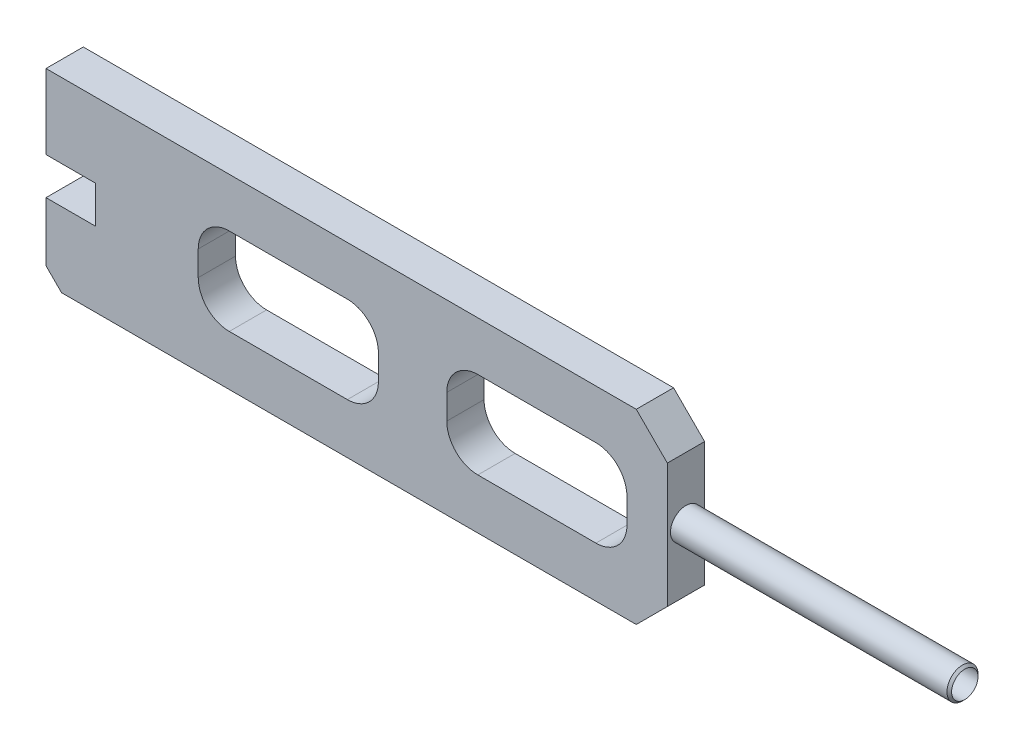
from build123d import *

# Parameters (mm, degrees)
SKETCH1_W              = 200
SKETCH1_H              = 60
BOSS_EXTRUDE1_DEPTH    = 12
SKETCH2_W              = 16
SKETCH2_H              = 12
CUT_EXTRUDE1_DEPTH     = 106.090437243
SKETCH3_W              = 58
SKETCH3_H              = 28
CUT_EXTRUDE2_DEPTH     = 106.090437243
SKETCH4_W              = 58
SKETCH4_H              = 28
CUT_EXTRUDE3_DEPTH     = 106.090437243
SKETCH5_W              = 90
SKETCH5_H              = 5
M6_TAPPED_HOLE1_D      = 5
M6_TAPPED_HOLE1_DEPTH  = 13
M6_TAPPED_HOLE1_TIP    = 1.502151548
CHAMFER1_SIZE          = 1
CHAMFER2_SIZE          = 10
CHAMFER3_SIZE          = 5
FILLET1_R              = 10
M10_TAPPED_HOLE1_D     = 8.5
M10_TAPPED_HOLE1_DEPTH = 99.5
M10_TAPPED_HOLE1_TIP   = 2.553657631


with BuildPart() as part:
    # Sketch1 → Boss-Extrude1 (new body)
    with BuildSketch(Plane.XY.offset(6)):
        Rectangle(SKETCH1_W, SKETCH1_H)
    extrude(amount=-BOSS_EXTRUDE1_DEPTH)

    # Sketch2 → Cut-Extrude1 (cut, through all)
    with BuildSketch(Plane(origin=(0, 0, -6), x_dir=(-1, 0, 0), z_dir=(0, 0, -1))):
        with Locations((92, 0)):
            Rectangle(SKETCH2_W, SKETCH2_H)
    extrude(amount=-CUT_EXTRUDE1_DEPTH, mode=Mode.SUBTRACT)

    # Sketch3 → Cut-Extrude2 (cut, through all)
    with BuildSketch(Plane.XY.offset(6)):
        with Locations((-22, 0.2)):
            Rectangle(SKETCH3_W, SKETCH3_H)
    extrude(amount=-CUT_EXTRUDE2_DEPTH, mode=Mode.SUBTRACT)

    # Sketch4 → Cut-Extrude3 (cut, through all)
    with BuildSketch(Plane(origin=(0, 0, -6), x_dir=(-1, 0, 0), z_dir=(0, 0, -1))):
        with Locations((-58, 0.2)):
            Rectangle(SKETCH4_W, SKETCH4_H)
    extrude(amount=-CUT_EXTRUDE3_DEPTH, mode=Mode.SUBTRACT)

    # Sketch5 → Revolve1 (revolve)
    with BuildSketch(Plane(origin=(0, 0, 0), x_dir=(-1, 0, 0), z_dir=(0, 0, -1)), mode=Mode.PRIVATE) as revolve1_sk:
        with Locations((-145, 2.7)):
            Rectangle(SKETCH5_W, SKETCH5_H)
    revolve(revolve1_sk.sketch.rotate(Axis((190, 0.2, 0), (-1, 0, 0)), 270), axis=Axis((190, 0.2, 0), (-1, 0, 0)))

    # M6 Tapped Hole1
    with Locations(Plane.ZY.offset(100)):
        with Locations((0, 18)):
            Hole(M6_TAPPED_HOLE1_D / 2, depth=M6_TAPPED_HOLE1_DEPTH)
            with Locations((0, 0, -(M6_TAPPED_HOLE1_DEPTH + M6_TAPPED_HOLE1_TIP / 2))):  # 118° drill point
                Cone(0, M6_TAPPED_HOLE1_D / 2, M6_TAPPED_HOLE1_TIP, mode=Mode.SUBTRACT)

    # Chamfer1
    chamfer1_edges = [part.edges().sort_by_distance(p)[0] for p in [
        (190, 0.2, -5),
    ]]
    chamfer(chamfer1_edges, length=CHAMFER1_SIZE)

    # Chamfer2
    chamfer2_edges = [part.edges().sort_by_distance(p)[0] for p in [
        (100, 30, 0),
        (100, -30, 0),
    ]]
    chamfer(chamfer2_edges, length=CHAMFER2_SIZE)

    # Chamfer3
    chamfer3_edges = [part.edges().sort_by_distance(p)[0] for p in [
        (-100, -30, 0),
    ]]
    chamfer(chamfer3_edges, length=CHAMFER3_SIZE)

    # Fillet1
    fillet1_edges = [part.edges().sort_by_distance(p)[0] for p in [
        (-51, -13.8, 0),
        (-51, 14.2, 0),
        (7, 14.2, 0),
        (7, -13.8, 0),
        (29, 14.2, 0),
        (29, -13.8, 0),
        (87, -13.8, 0),
        (87, 14.2, 0),
    ]]
    fillet(fillet1_edges, radius=FILLET1_R)

    # M10 Tapped Hole1
    with Locations(Plane(origin=(190, 0, 0), x_dir=(0, 0, -1), z_dir=(1, 0, 0))):
        with Locations((0, 0.2)):
            Hole(M10_TAPPED_HOLE1_D / 2, depth=M10_TAPPED_HOLE1_DEPTH)
            with Locations((0, 0, -(M10_TAPPED_HOLE1_DEPTH + M10_TAPPED_HOLE1_TIP / 2))):  # 118° drill point
                Cone(0, M10_TAPPED_HOLE1_D / 2, M10_TAPPED_HOLE1_TIP, mode=Mode.SUBTRACT)


solid = part.part
